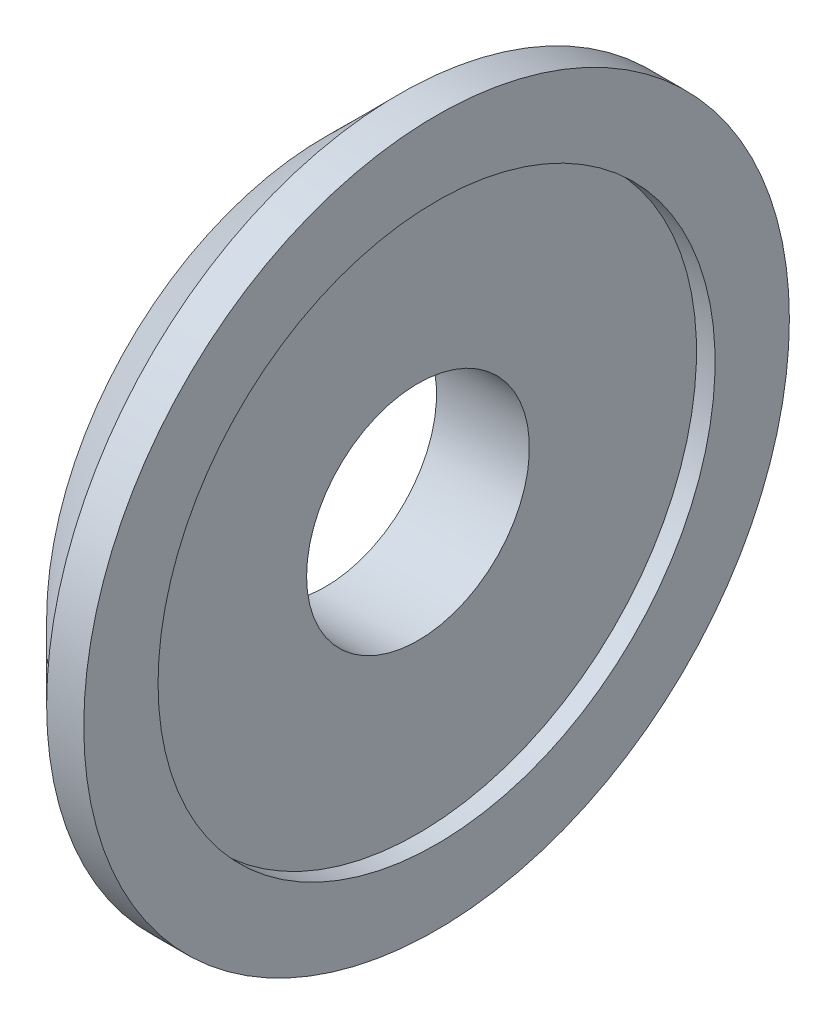
SolidWorks part; units mm, degrees
ref_plane "Front Plane" through (0, 0, 0) normal (0, 0, 1) x (1, 0, 0)
ref_plane "Top Plane" through (0, 0, 0) normal (0, 1, 0) x (1, 0, 0)
ref_plane "Right Plane" through (0, 0, 0) normal (1, 0, 0) x (0, 0, -1)
sketch "Sketch1" plane through (0, 0, 0) normal (0, 0, 1) x (1, 0, 0)
  line L0 (-11.2599, 0) -> (14.6484, 0) construction
  line L2 (-3, 15) -> (-3, 6)
  line L4 (3, 19) -> (3, 15)
  line L5 (-3, 6) -> (2, 6)
  line L6 (2, 15) -> (2, 6)
  line L7 (2, 15) -> (3, 15)
  line L8 (3, 19) -> (1, 19)
  line L10 (1, 19) -> (-3, 15)
  point P0 (0, 0)
  dimension "D1" = 2
  dimension "D2" = 19
  dimension "D3" = 6
  dimension "D4" = 15
  dimension "D5" = 1
revolve "Revolve2" add sketch "Sketch1" angle 360 about L0
